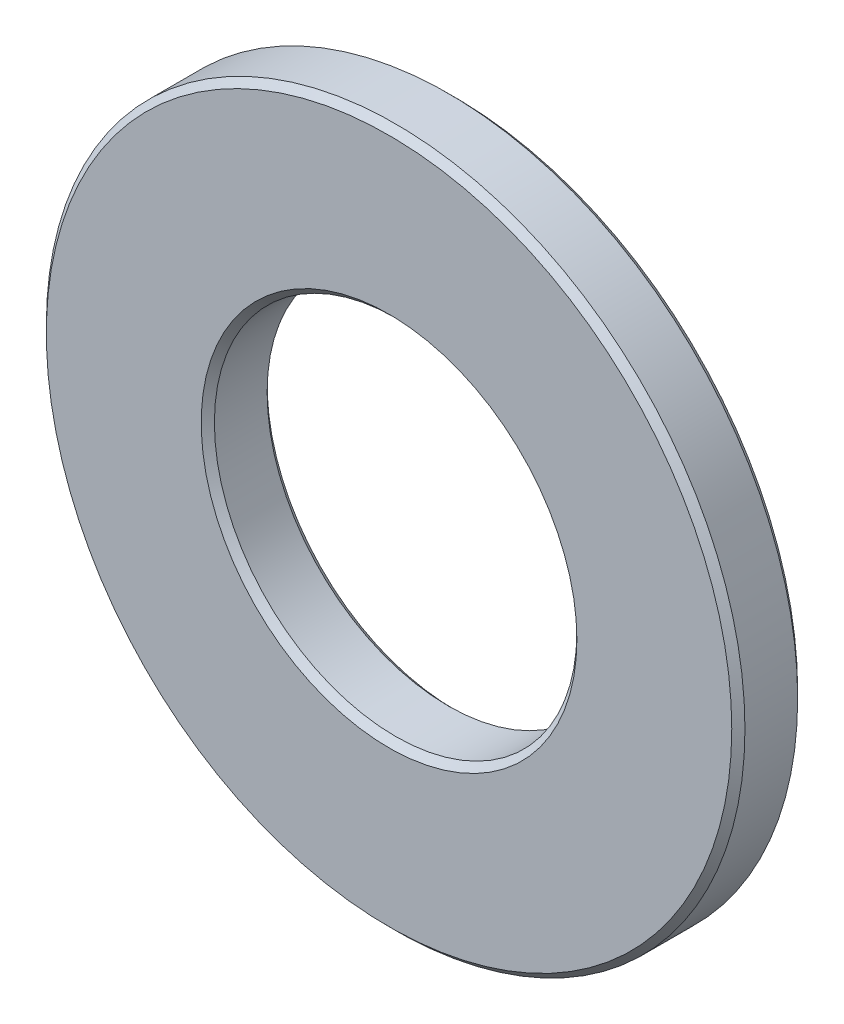
from build123d import *

# Parameters (mm, degrees)
SKETCH1_R           = 53
SKETCH1_R_2         = 27.5
BOSS_EXTRUDE1_DEPTH = 10
CHAMFER1_SIZE       = 1


with BuildPart() as part:
    # Sketch1 → Boss-Extrude1 (new body)
    with BuildSketch(Plane.XY):
        Circle(SKETCH1_R)
        Circle(SKETCH1_R_2, mode=Mode.SUBTRACT)
    extrude(amount=BOSS_EXTRUDE1_DEPTH)

    # Chamfer1
    chamfer1_edges = [part.edges().sort_by_distance(p)[0] for p in [
        (-53, 0, 0),
        (-53, 0, 10),
        (-27.5, 0, 0),
        (-27.5, 0, 10),
    ]]
    chamfer(chamfer1_edges, length=CHAMFER1_SIZE)


solid = part.part
